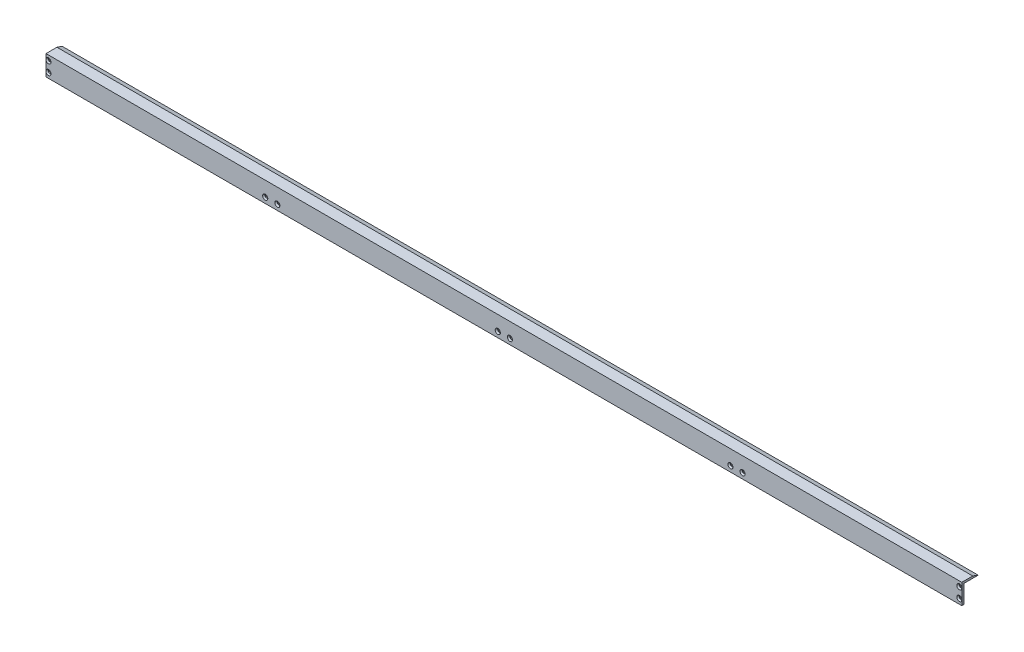
from build123d import *

# Parameters (mm, degrees)
SKETCH1_W                                            = 2260
SKETCH1_H                                            = 50
BOSS_EXTRUDE1_DEPTH                                  = 5
BOSS_EXTRUDE2_DEPTH                                  = 2260
CSK_FOR_M6_HEXAGON_LOBULAR_SOCKET_RAISED_D           = 6.6
CSK_FOR_M6_HEXAGON_LOBULAR_SOCKET_RAISED_DEPTH       = 19.75
CSK_FOR_M6_HEXAGON_LOBULAR_SOCKET_RAISED_CSINK_D     = 12.8
CSK_FOR_M6_HEXAGON_LOBULAR_SOCKET_RAISED_CSINK_ANGLE = 90
CSK_FOR_M6_HEXAGON_LOBULAR_SOCKET_RAISED_TIP         = 1.982840043


with BuildPart() as part:
    # Sketch1 → Boss-Extrude1 (new body)
    with BuildSketch(Plane.XY):
        Rectangle(SKETCH1_W, SKETCH1_H)
    extrude(amount=BOSS_EXTRUDE1_DEPTH)

    # Sketch2 → Boss-Extrude2 (add)
    with BuildSketch(Plane.ZY.offset(1130)):
        Polygon((0, 25), (-22, 25), (-35, 20.5), (-35, 20), (0, 20), align=None)
    extrude(amount=-BOSS_EXTRUDE2_DEPTH)

    # CSK for M6 Hexagon lobular socket raised CTSK head screws1
    with Locations(Plane.XY.offset(5)):
        with Locations((-589, -11.306794409), (-559, -11.306794409), (-15, -11.306794409), (15, -11.306794409), (559, -11.306794409), (589, -11.306794409), (-1124, -12.5), (-1124, 12.5), (1124, -12.5), (1124, 12.5)):
            CounterSinkHole(CSK_FOR_M6_HEXAGON_LOBULAR_SOCKET_RAISED_D / 2, CSK_FOR_M6_HEXAGON_LOBULAR_SOCKET_RAISED_CSINK_D / 2, depth=CSK_FOR_M6_HEXAGON_LOBULAR_SOCKET_RAISED_DEPTH, counter_sink_angle=CSK_FOR_M6_HEXAGON_LOBULAR_SOCKET_RAISED_CSINK_ANGLE)
            with Locations((0, 0, -(CSK_FOR_M6_HEXAGON_LOBULAR_SOCKET_RAISED_DEPTH + CSK_FOR_M6_HEXAGON_LOBULAR_SOCKET_RAISED_TIP / 2))):  # 118° drill point
                Cone(0, CSK_FOR_M6_HEXAGON_LOBULAR_SOCKET_RAISED_D / 2, CSK_FOR_M6_HEXAGON_LOBULAR_SOCKET_RAISED_TIP, mode=Mode.SUBTRACT)


solid = part.part
